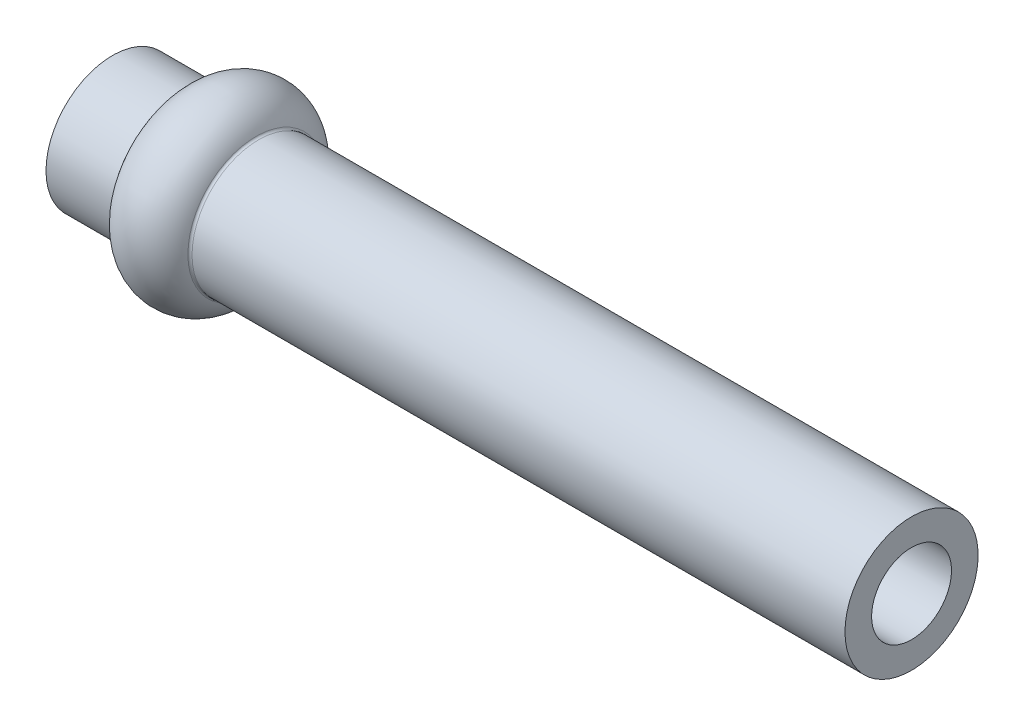
from build123d import *

# Parameters (mm, degrees)
FILLET1_R = 0.1


with BuildPart() as part:
    # Sketch1 → Revolve1 (revolve)
    with BuildSketch(Plane.XY, mode=Mode.PRIVATE) as revolve1_sk:
        with BuildLine():
            Line((0, 2.5), (2.585786438, 2.5))
            ThreePointArc((2.585786438, 2.5), (4, 3.5), (5.414213562, 2.5))
            Line((5.414213562, 2.5), (30, 2.5))
            Line((30, 2.5), (30, 1.5))
            Line((30, 1.5), (0, 1.5))
            Line((0, 1.5), (0, 2.5))
        make_face()
    revolve(revolve1_sk.sketch.rotate(Axis((0, 0, 0), (1, 0, 0)), 90), axis=Axis((0, 0, 0), (1, 0, 0)))

    # Fillet1
    fillet1_edges = [part.edges().sort_by_distance(p)[0] for p in [
        (2.585786438, 0, -2.5),
        (5.414213562, 0, -2.5),
    ]]
    fillet(fillet1_edges, radius=FILLET1_R)


solid = part.part
